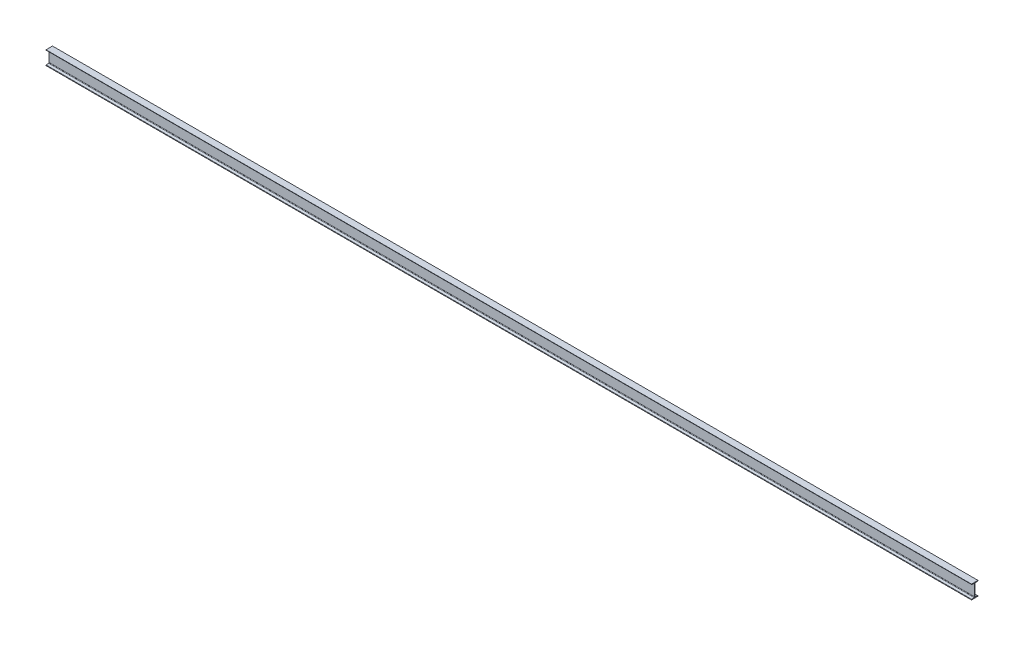
SolidWorks part; units mm, degrees
ref_plane "Front" through (0, 0, 0) normal (0, 0, 1) x (1, 0, 0)
ref_plane "Top" through (0, 0, 0) normal (0, 1, 0) x (1, 0, 0)
ref_plane "Right" through (0, 0, 0) normal (1, 0, 0) x (0, 0, -1)
other "Configuration Table"
sketch "Sketch1" plane through (0, 0, 0) normal (1, 0, 0) x (0, 0, -1)
  line L0 (-59, 0) -> (59, 0)
  line L1 (0, 106.3348) -> (0, -35.2641) construction
  line L2 (-5, 233.3333) -> (-5, 16.6667)
  line L3 (-5, 16.6667) -> (-59, 7.6667)
  line L4 (-59, 7.6667) -> (-59, 0)
  line L5 (-59, 7.6667) -> (-5, 7.6667) construction
  line L6 (-5, 7.6667) -> (-5, 16.6667) construction
  line L7 (-27, 250) -> (-27, 0) construction
  line L8 (-59, 250) -> (59, 250)
  line L9 (-59, 250) -> (-59, 242.3333)
  line L10 (-59, 242.3333) -> (-5, 233.3333)
  line L11 (-59, 242.3333) -> (-5, 242.3333) construction
  line L12 (-5, 242.3333) -> (-5, 233.3333) construction
  line L13 (-27, 13) -> (-27, 0) construction
  line L14 (-27, 250) -> (-27, 237) construction
  line L15 (59, 7.6667) -> (59, 0)
  line L16 (5, 16.6667) -> (59, 7.6667)
  line L17 (5, 233.3333) -> (5, 16.6667)
  line L18 (59, 242.3333) -> (5, 233.3333)
  line L19 (59, 250) -> (59, 242.3333)
  point P22 (0, 250)
extrude "Base" add sketch "Sketch1" along normal blind 16840
fillet "Fillet1" radius 10 4 edges at (8420, 233.3333, -5) (8420, 16.6667, -5) (8420, 16.6667, 5) (8420, 233.3333, 5)
fillet "Fillet2" radius 5 4 edges at (8420, 242.3333, 59) (8420, 7.6667, 59) (8420, 7.6667, -59) (8420, 242.3333, -59)
equation "\"D5@Sketch1\" =  ( \"b@Sketch1\" - \"d@Sketch1\" ) /12"
equation "\"D10@Sketch1\" = \"D5@Sketch1\""
equation "\"t1@Sketch1\" = \"t@Sketch1\""
equation "\"D6@Sketch1\" =  ( \"b@Sketch1\" - \"d@Sketch1\" ) /4"
